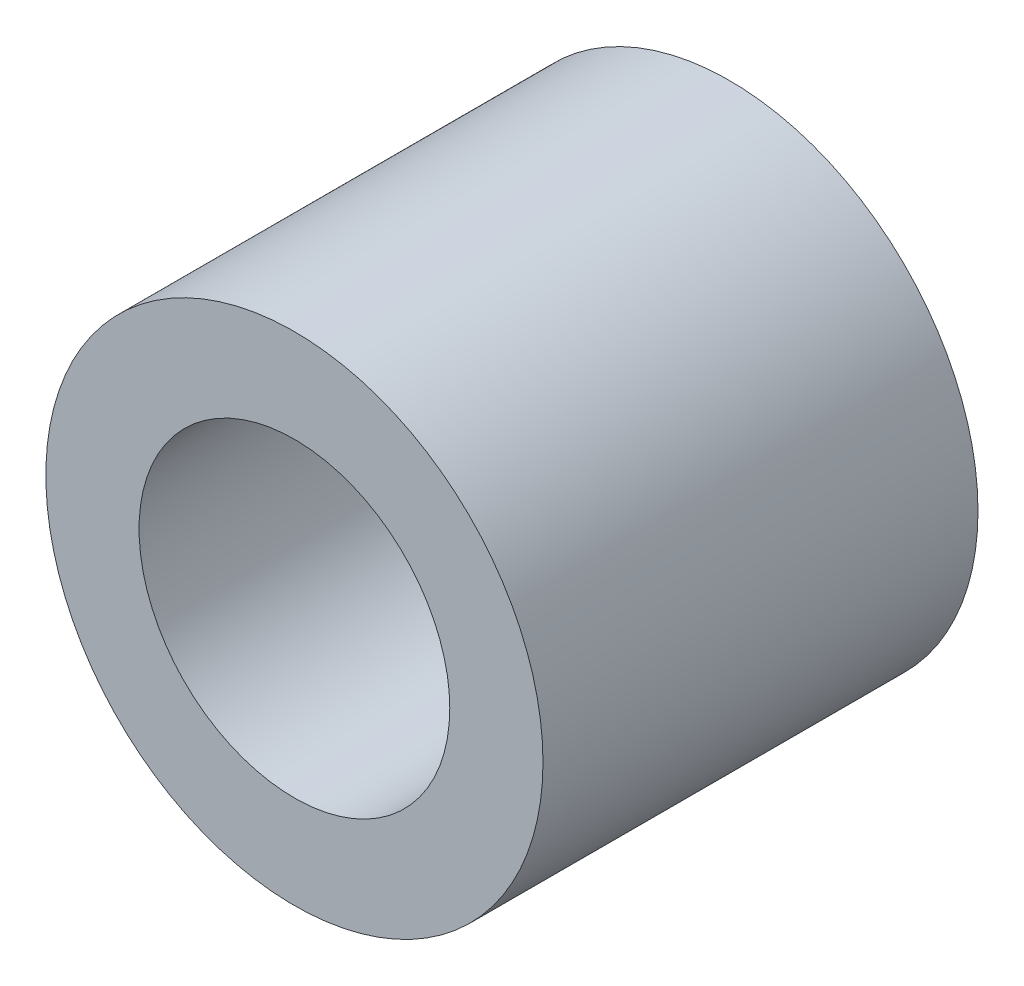
SolidWorks part; units mm, degrees
ref_plane "前视基准面" through (0, 0, 0) normal (0, 0, 1) x (1, 0, 0)
ref_plane "上视基准面" through (0, 0, 0) normal (0, 1, 0) x (1, 0, 0)
ref_plane "右视基准面" through (0, 0, 0) normal (1, 0, 0) x (0, 0, -1)
sketch "草图1" plane through (0, 0, 0) normal (0, 0, 1) x (1, 0, 0)
  circle A0 centre (0, 0) radius 2.5
  circle A1 centre (0, 0) radius 4
  dimension "D1" = 5
  dimension "D2" = 8
extrude "凸台-拉伸1" add sketch "草图1" along normal blind 7
